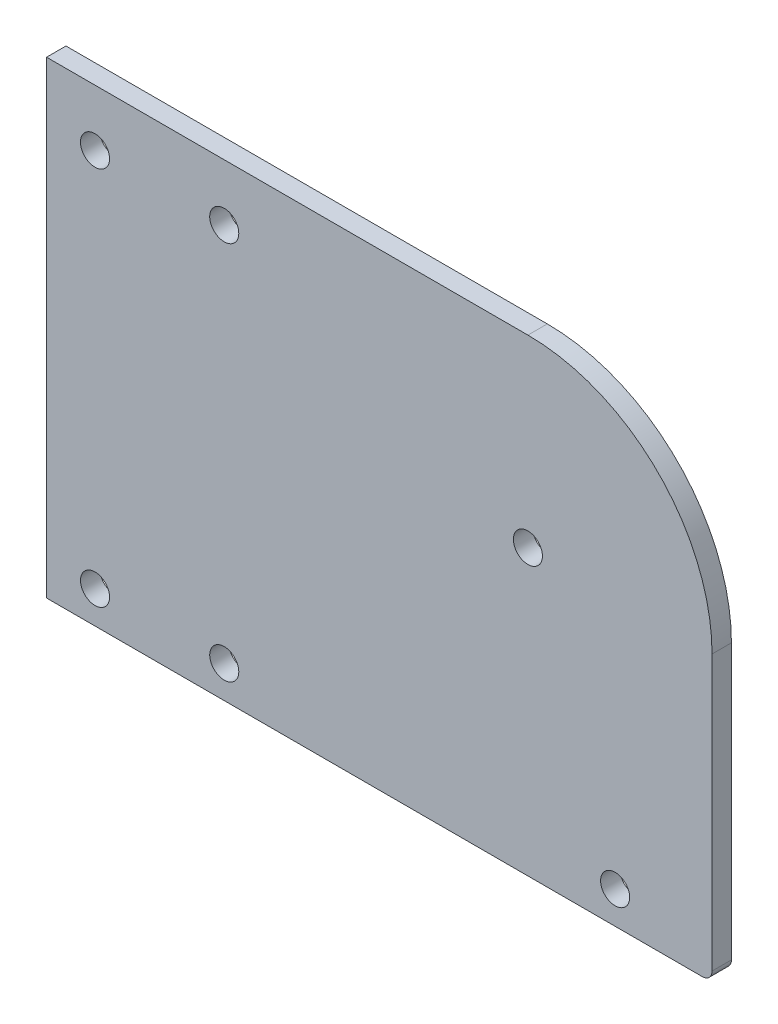
from build123d import *

# Parameters (mm, degrees)
SKETCH_1_W          = 206
SKETCH_1_H          = 145
EXTRUDE_1_DEPTH     = 6
SKETCH_3_R          = 4.5
CUT_EXTRUDE_2_DEPTH = 127.100158604
SKETCH_4_R          = 4.5
CUT_EXTRUDE_3_DEPTH = 127.100158604
FILLET_4_R          = 57
SKETCH_10_R         = 4.5
CUT_EXTRUDE_6_DEPTH = 10
FILLET_6_R          = 3


with BuildPart() as part:
    # 草图1 → 凸台-拉伸1 (new body)
    with BuildSketch(Plane.XY):
        Rectangle(SKETCH_1_W, SKETCH_1_H)
    extrude(amount=EXTRUDE_1_DEPTH)

    # 草图3 → 切除-拉伸2 (cut, through all)
    with BuildSketch(Plane.XY.offset(6)):
        with Locations((-88, 55)):
            Circle(SKETCH_3_R)
        with Locations((-48, 55)):
            Circle(SKETCH_3_R)
        with Locations((-88, -62.5)):
            Circle(SKETCH_3_R)
        with Locations((-48, -62.5)):
            Circle(SKETCH_3_R)
    extrude(amount=-CUT_EXTRUDE_2_DEPTH, mode=Mode.SUBTRACT)

    # 草图4 → 切除-拉伸3 (cut, through all)
    with BuildSketch(Plane.XY.offset(6)):
        with Locations((46, 15.5)):
            Circle(SKETCH_4_R)
    extrude(amount=-CUT_EXTRUDE_3_DEPTH, mode=Mode.SUBTRACT)

    # 圆角4
    fillet_4_edges = [part.edges().sort_by_distance(p)[0] for p in [
        (103, 72.5, 3),
    ]]
    fillet(fillet_4_edges, radius=FILLET_4_R)

    # 草图10 → 切除-拉伸6 (cut)
    with BuildSketch(Plane(origin=(0, 0, 0), x_dir=(-1, 0, 0), z_dir=(0, 0, -1))):
        with Locations((-73, -62.5)):
            Circle(SKETCH_10_R)
    extrude(amount=-CUT_EXTRUDE_6_DEPTH, mode=Mode.SUBTRACT)

    # 圆角6
    fillet_6_edges = [part.edges().sort_by_distance(p)[0] for p in [
        (103, -72.5, 3),
    ]]
    fillet(fillet_6_edges, radius=FILLET_6_R)


solid = part.part
